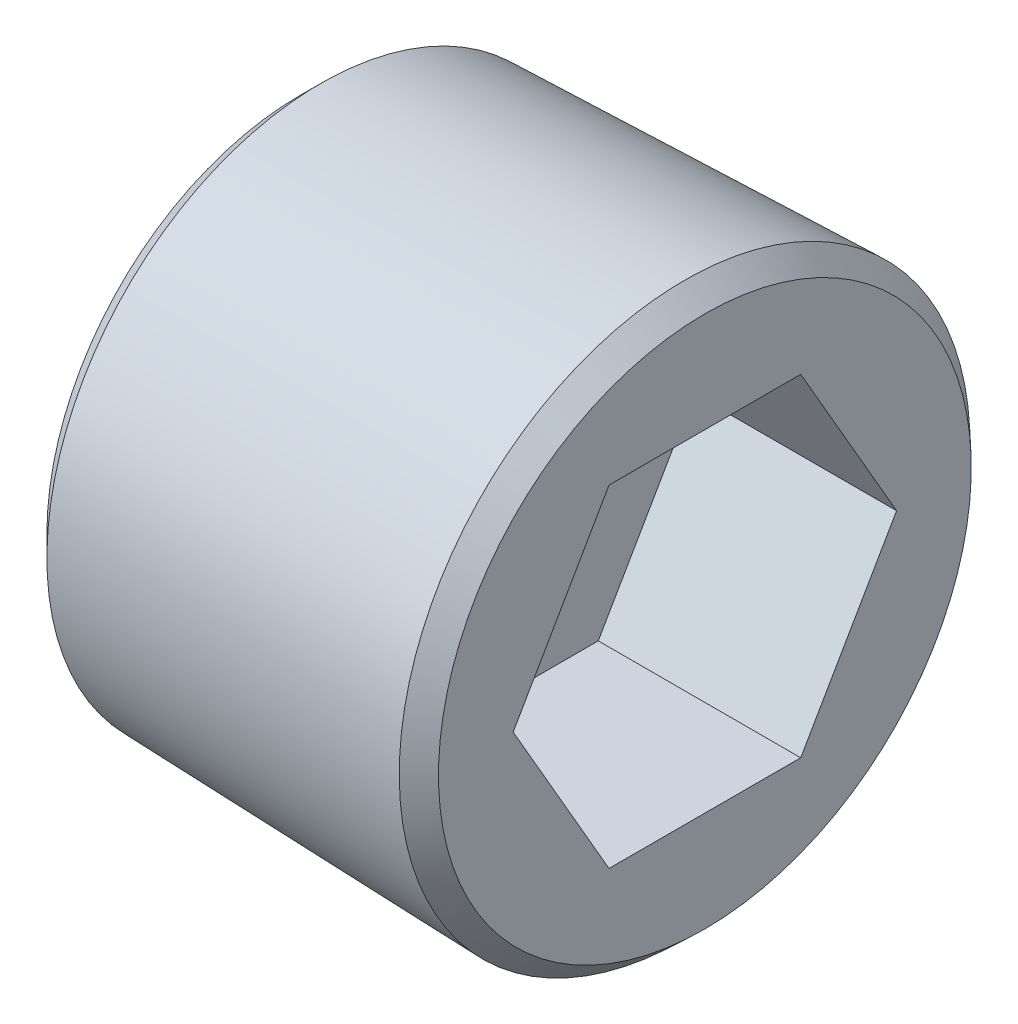
from build123d import *
from OCP.BRepFilletAPI import BRepFilletAPI_MakeChamfer

# Parameters (mm, degrees)
CUT_EXTRUDE_1_DEPTH = 5
CHAMFER_1_SIZE      = 0.5
CHAMFER_1_SIZE2     = 0.516477811
CHAMFER_1_SIZE2_2   = 0.485004947


with BuildPart() as part:
    # 草图1 → 旋转1 (revolve)
    with BuildSketch(Plane.XY):
        Polygon((0, 0), (0, 6.75), (10, 7.06426266), (10, 0), align=None)
    revolve(axis=Axis((0, 0, 0), (-1, 0, 0)))

    # 草图2 → 切除-拉伸1 (cut)
    with BuildSketch(Plane(origin=(10, 0, 0), x_dir=(0, 0, -1), z_dir=(1, 0, 0))):
        Polygon((2.367136104, -4.1), (4.734272207, 0), (2.367136104, 4.1), (-2.367136104, 4.1), (-4.734272207, 0), (-2.367136104, -4.1), align=None)
    extrude(amount=-CUT_EXTRUDE_1_DEPTH, mode=Mode.SUBTRACT)

    # 倒角1: one chamfer whose edges measure the first distance from different faces: ONE call of the kernel's chamfer builder (chamfer() names one face for all edges)
    chamfer_1_edges_1 = [part.edges().sort_by_distance(p)[0] for p in [
        (0, -6.75, 0),
    ]]
    chamfer_1_side_1 = [part.faces().sort_by_distance(p)[0] for p in [
        (0, 0, 0),
    ]]
    chamfer_1_edges_2 = [part.edges().sort_by_distance(p)[0] for p in [
        (10, -7.06426266, 0),
    ]]
    chamfer_1_side_2 = [part.faces().sort_by_distance(p)[0] for p in [
        (5, -6.90713133, 0),
    ]]
    chamfer_1 = BRepFilletAPI_MakeChamfer(part.part.solid().wrapped)
    for e in chamfer_1_edges_1:
        chamfer_1.Add(CHAMFER_1_SIZE, CHAMFER_1_SIZE2, e.wrapped, chamfer_1_side_1[0].wrapped)  # the first distance lies on this face
    for e in chamfer_1_edges_2:
        chamfer_1.Add(CHAMFER_1_SIZE, CHAMFER_1_SIZE2_2, e.wrapped, chamfer_1_side_2[0].wrapped)  # the first distance lies on this face
    add(Compound.cast(chamfer_1.Shape()), mode=Mode.REPLACE)


solid = part.part
